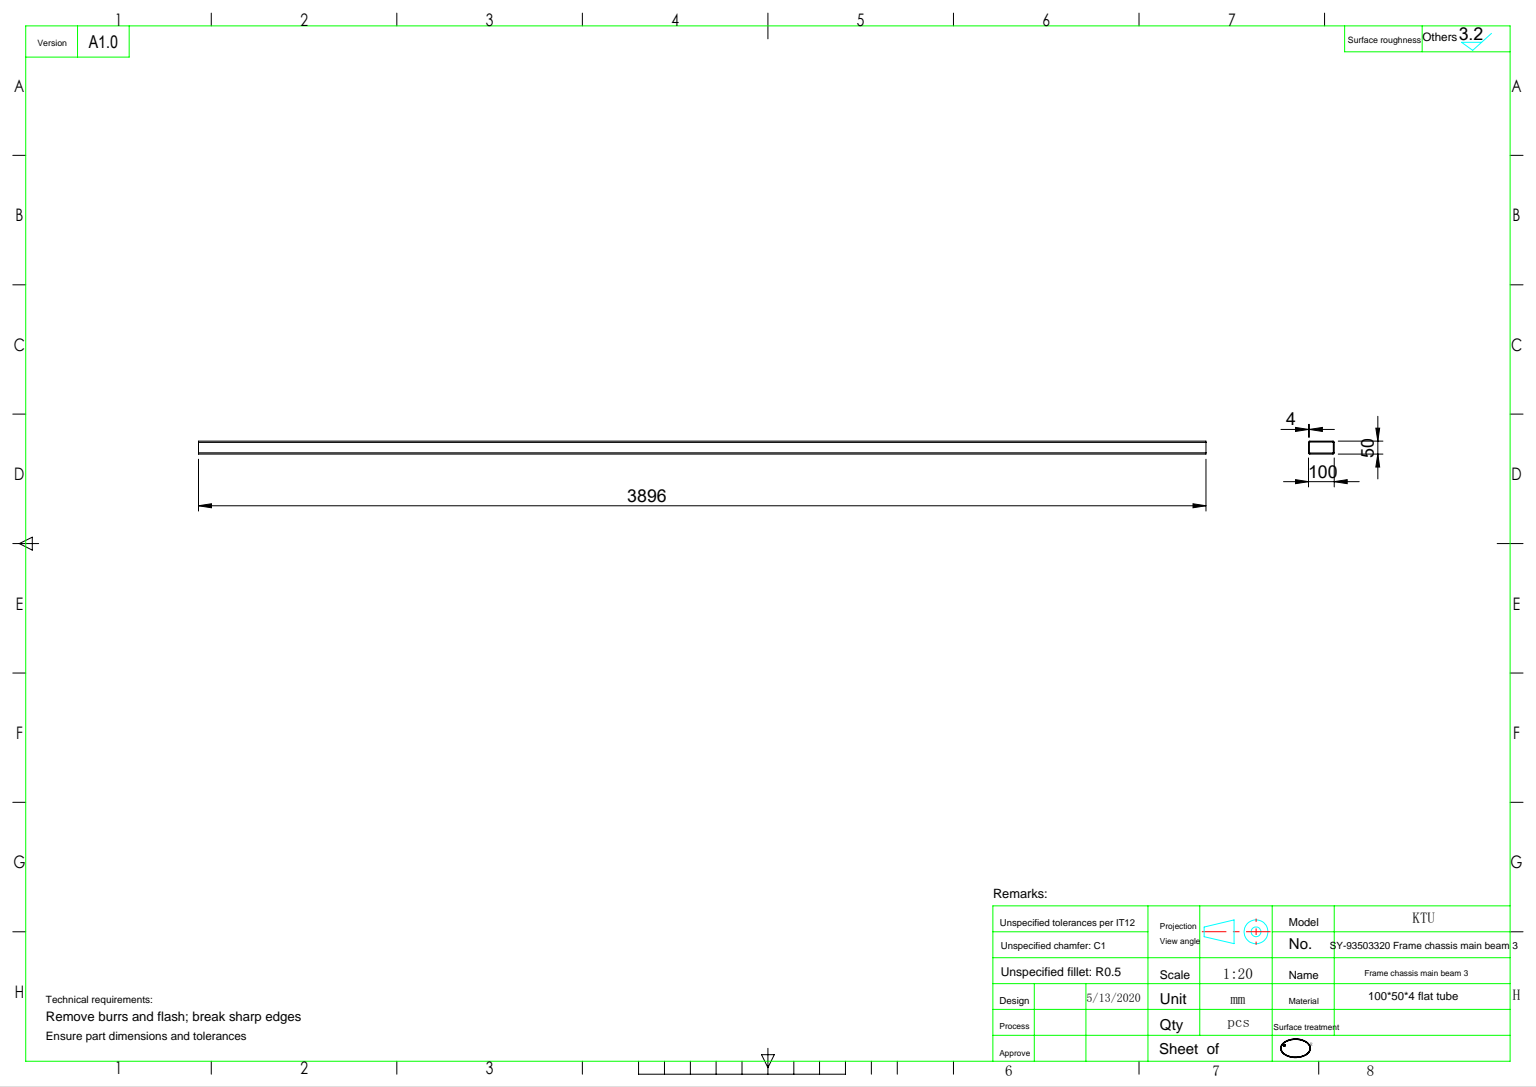
from build123d import *

# Parameters (mm, degrees)
EXTRUDE_1_DEPTH = 1948


with BuildPart() as part:
    # 草图1 → 拉伸-薄壁1 (new, symmetric)
    with BuildSketch(Plane.XY):
        with BuildLine():
            Line((-45, 25), (45, 25))
            ThreePointArc((45, 25), (48.535533906, 23.535533906), (50, 20))
            Line((50, 20), (50, -20))
            ThreePointArc((50, -20), (48.535533906, -23.535533906), (45, -25))
            Line((45, -25), (-45, -25))
            ThreePointArc((-45, -25), (-48.535533906, -23.535533906), (-50, -20))
            Line((-50, -20), (-50, 20))
            ThreePointArc((-50, 20), (-48.535533906, 23.535533906), (-45, 25))
        make_face()
        with BuildLine():
            Line((-45, 21), (45, 21))
            ThreePointArc((45, 21), (45.707106781, 20.707106781), (46, 20))
            Line((46, 20), (46, -20))
            ThreePointArc((46, -20), (45.707106781, -20.707106781), (45, -21))
            Line((45, -21), (-45, -21))
            ThreePointArc((-45, -21), (-45.707106781, -20.707106781), (-46, -20))
            Line((-46, -20), (-46, 20))
            ThreePointArc((-46, 20), (-45.707106781, 20.707106781), (-45, 21))
        make_face(mode=Mode.SUBTRACT)
    extrude(amount=EXTRUDE_1_DEPTH, both=True)


solid = part.part
